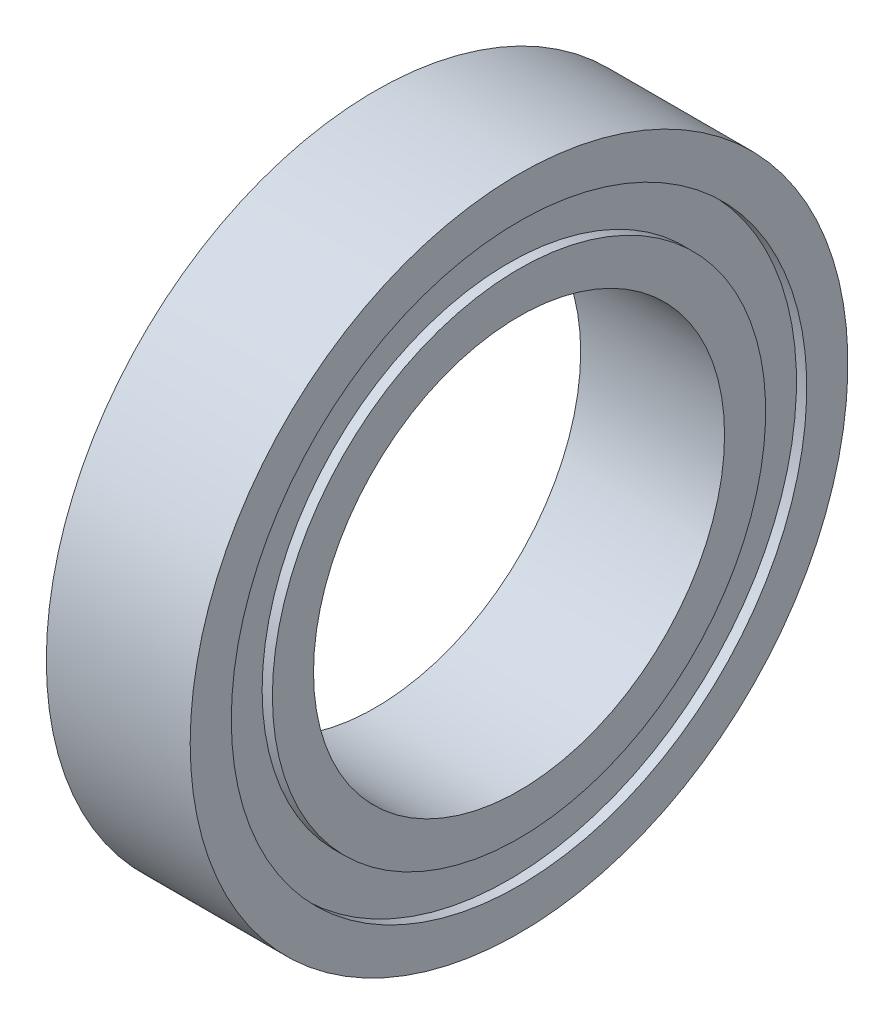
from build123d import *


with BuildPart() as part:
    # Sketch1 → Revolve1 (revolve)
    with BuildSketch(Plane.XY, mode=Mode.PRIVATE) as revolve1_sk:
        Polygon((14.644406169, 14), (14.644406169, 16), (21.644406169, 16), (21.644406169, 14), (21.144406169, 14), (21.144406169, 12), (21.644406169, 12), (21.644406169, 10), (14.644406169, 10), (14.644406169, 12), (15.144406169, 12), (15.144406169, 14), align=None)
    revolve(revolve1_sk.sketch.rotate(Axis((0, 0, 0), (1, 0, 0)), 90), axis=Axis((0, 0, 0), (1, 0, 0)))


solid = part.part
